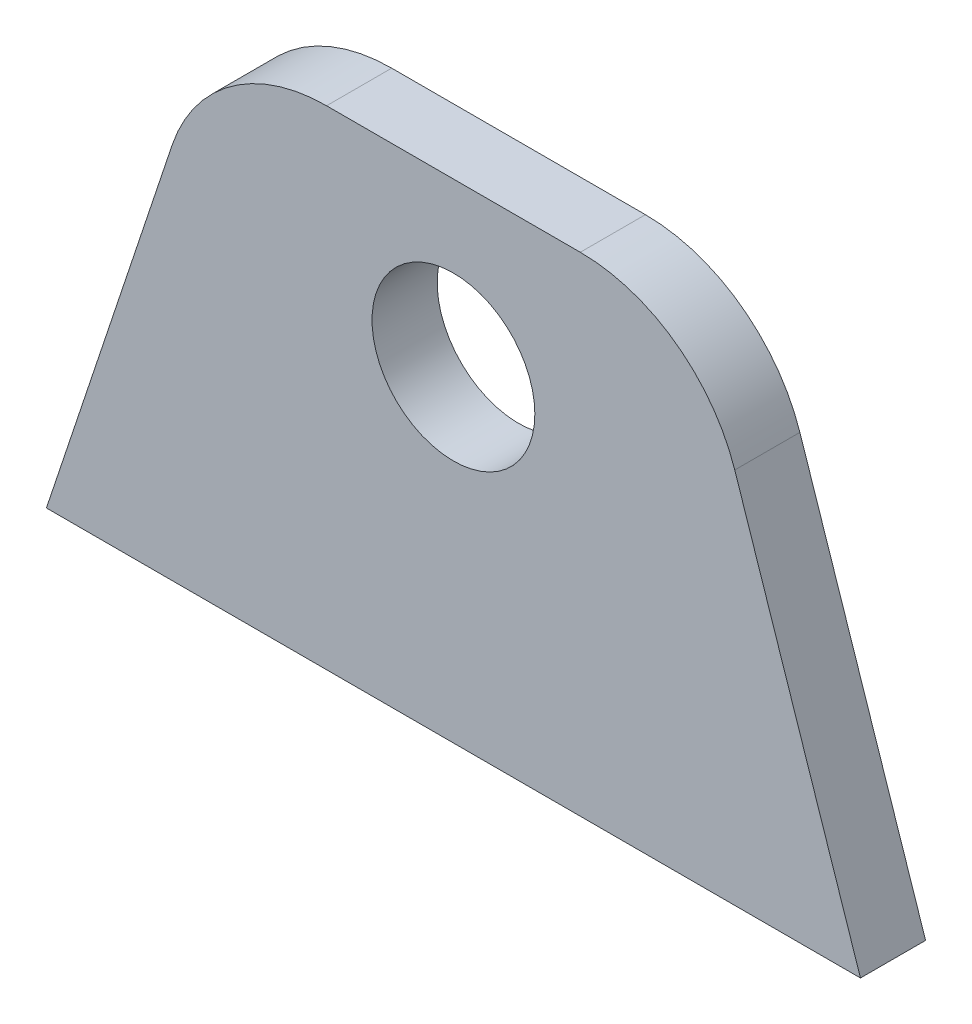
SolidWorks part; units mm, degrees
material "1023 碳钢板 (SS)"
ref_plane "Front Plane" through (0, 0, 0) normal (0, 0, 1) x (1, 0, 0)
ref_plane "Top Plane" through (0, 0, 0) normal (0, 1, 0) x (1, 0, 0)
ref_plane "Right Plane" through (0, 0, 0) normal (1, 0, 0) x (0, 0, -1)
sketch "Sketch1" plane through (0, 0, 0) normal (0, 0, 1) x (1, 0, 0)
  line L0 (0, 0) -> (50, 0)
  line L1 (50, 0) -> (42.2792, 23.1623)
  line L2 (32.7924, 30) -> (17.2076, 30)
  line L3 (7.7208, 23.1623) -> (0, 0)
  arc A0 (42.2792, 23.1623) -> (32.7924, 30) centre (32.7924, 20) ccw
  arc A1 (17.2076, 30) -> (7.7208, 23.1623) centre (17.2076, 20) ccw
  circle A2 centre (25, 20) radius 5
  point P7 (40, 30)
  point P10 (10, 30)
  point P14 (25, 0)
  dimension "D4" = 10
  dimension "D5" = 10
  dimension "D1" = 50
  dimension "D2" = 30
  dimension "D3" = 30
  dimension "D6" = 20
extrude "Boss-Extrude1" add sketch "Sketch1" along normal blind 4
